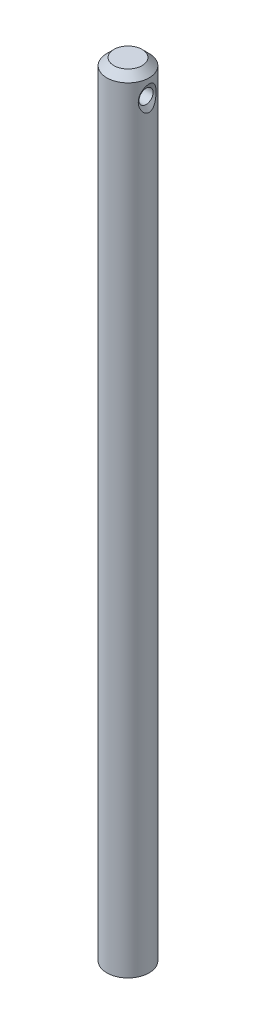
from build123d import *

# Parameters (mm, degrees)
SKETCH1_R               = 3
BOSS_EXTRUDE1_DEPTH     = 111
CUT_EXTRUDE1_DEPTH      = 112.081051489
CUT_EXTRUDE1_DEPTH_BACK = 112.081051489
SKETCH2_R               = 1
CHAMFER3_SIZE           = 1


with BuildPart() as part:
    # Sketch1 → Boss-Extrude1 (new body)
    with BuildSketch(Plane(origin=(0, 0, 0), x_dir=(1, 0, 0), z_dir=(0, 1, 0))):
        with Locations(Location((0, 0, 0), (0, 0, 270))):
            Circle(SKETCH1_R)
    extrude(amount=BOSS_EXTRUDE1_DEPTH)

    # Sketch2 → Cut-Extrude1 (cut, two sides: drawn at the far end of the back side and taken through both)
    with BuildSketch(Plane(origin=(0, 0, 0), x_dir=(0, 0, -1), z_dir=(1, 0, 0)).offset(-CUT_EXTRUDE1_DEPTH_BACK)):
        with Locations((0, 107.5)):
            Circle(SKETCH2_R)
    extrude(amount=CUT_EXTRUDE1_DEPTH + CUT_EXTRUDE1_DEPTH_BACK, mode=Mode.SUBTRACT)

    # Cut-Extrude2 cone 1 section (through the dimple's axis) → Cut-Extrude2 (revolve, cut)
    with BuildSketch(Plane(origin=(3, 107.5, 0), x_dir=(0, 0, -1), z_dir=(0, 1, 0))):
        Polygon((0, 0), (1.75, 0), (0, 1.010362971), align=None)
    cut_extrude2 = revolve(axis=Axis((3, 107.5, 0), (-1, 0, 0)), mode=Mode.SUBTRACT)

    # Mirror1: Cut-Extrude2 across plane
    add(cut_extrude2.mirror(Plane(origin=(0, 0, 0), x_dir=(0, 0, 1), z_dir=(1, 0, 0))), mode=Mode.SUBTRACT)

    # Chamfer3
    chamfer3_edges = [part.edges().sort_by_distance(p)[0] for p in [
        (0, 111, -3),
    ]]
    chamfer(chamfer3_edges, length=CHAMFER3_SIZE)


solid = part.part
